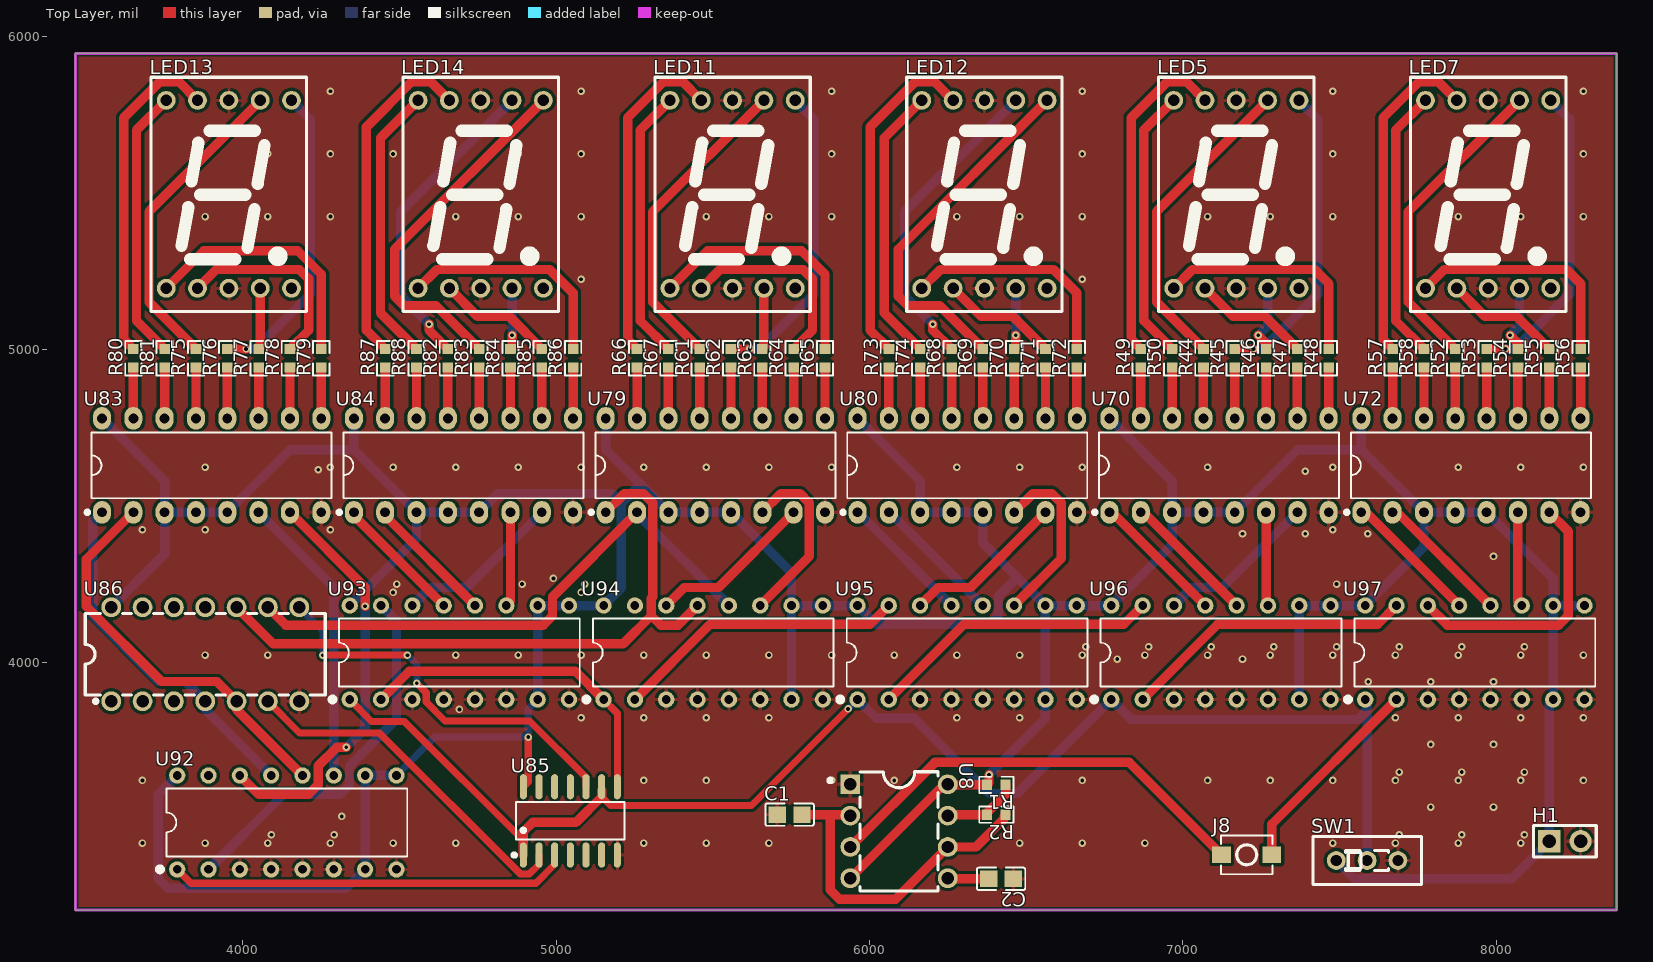
[diagram p0: Top Layer view]
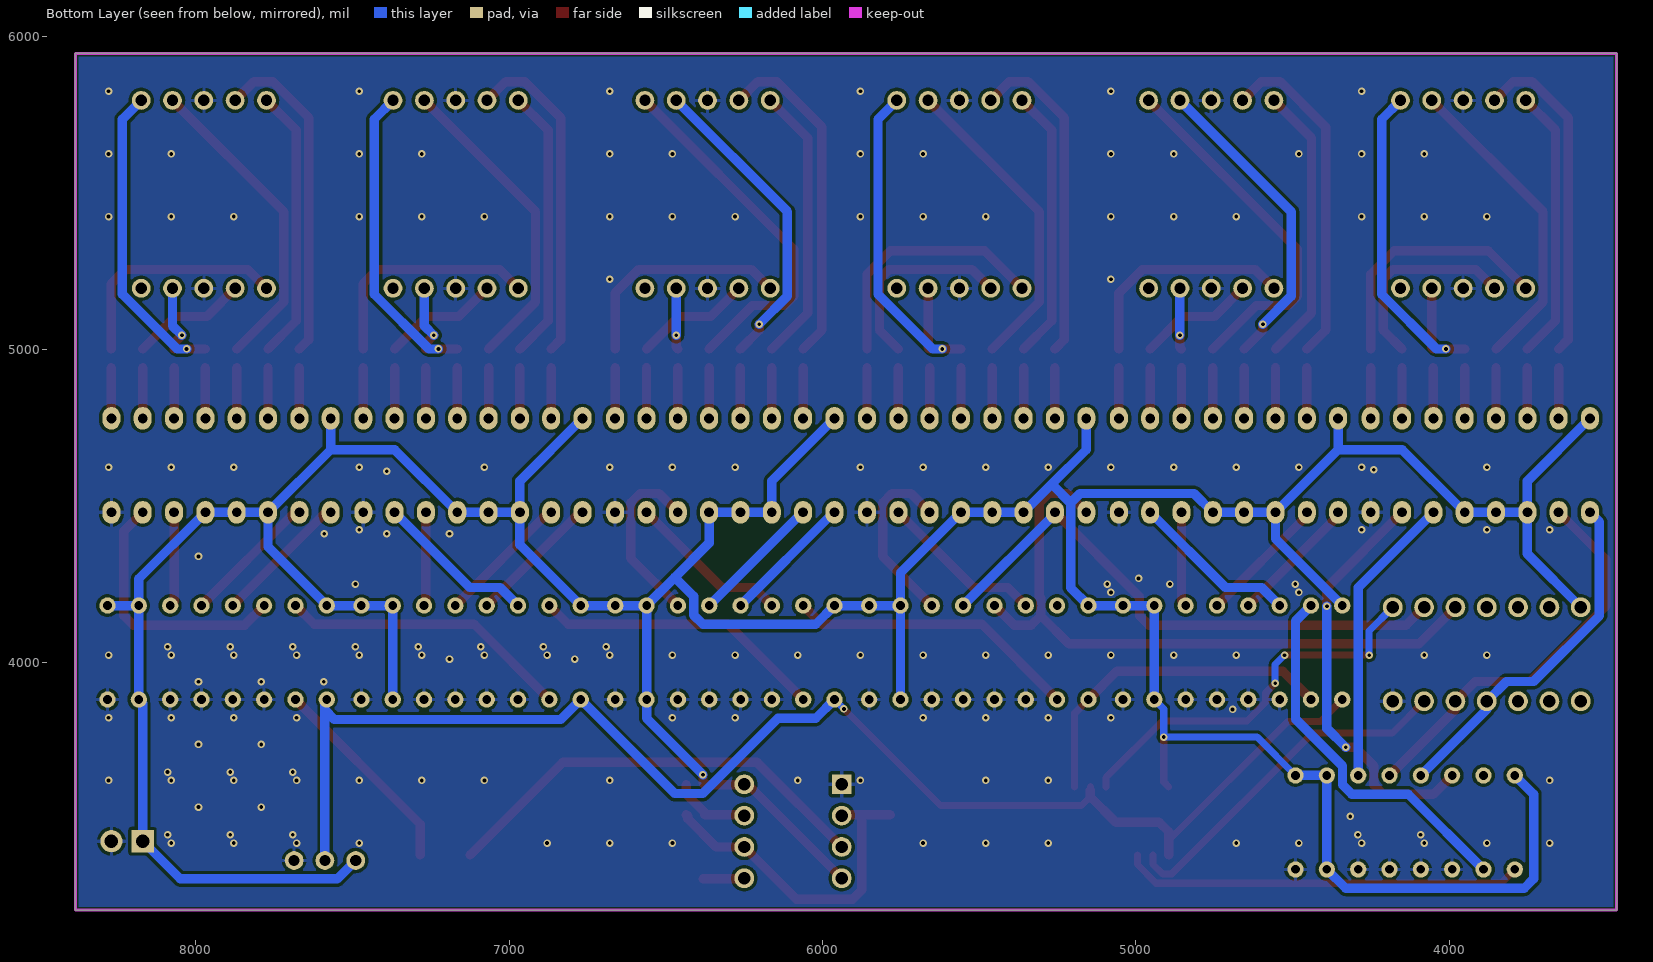
[diagram p1: Bottom Layer view, seen from below]
# Altium PCB MISC52151.pcbdoc
Units mil, origin at the board's own origin, x right, y up, seen from the top; angles counter-clockwise.
Board outline 4920 x 2735 mil, 2 copper layers (Top Layer, Bottom Layer), stack 62.206 mil thick; 70 components, 124 nets, 387 pads, 179 vias.

## Layer stack, top to bottom
Top Solder Mask Layer: solder mask 0.394, Dk 3.3
Top Layer: signal copper 1.379
Dielectric1: surface 59.449, FR4, Dk 4.5
Bottom Layer: signal copper 1.378
Bottom Solder Mask Layer: solder mask 0.394, Dk 3.3

## Board outline
3465,5945 3465,3210 8385,3210 8385,5945

## Design rules (kind name [scope] priority, off if disabled: settings)
BoardOutlineClearance copperThickness2oz_1 [All] p2 off: genericclearance=7.99 ignorepadtopadclearanceinfootprint=FALSE except(0: Arc-SplitContinuation Track-SplitContinuation SMDPad-SplitContinuation THPad-SplitContinuation Via-SplitContinuation Fill-SplitContinuation Region-SplitContinuation Poly-SplitContinuation Text-SplitContinuation Hole-SplitContinuation; 5.98: Arc-CutoutEdge Track-CutoutEdge SMDPad-CutoutEdge THPad-CutoutEdge Via-CutoutEdge Text-CutoutEdge; 6.89: Hole-OutlineEdge Hole-CutoutEdge; 10: Poly-OutlineEdge Poly-CutoutEdge; 11.81: Arc-OutlineEdge Track-OutlineEdge SMDPad-OutlineEdge THPad-OutlineEdge Via-OutlineEdge Fill-OutlineEdge Region-OutlineEdge Text-OutlineEdge Fill-CutoutEdge Region-CutoutEdge)
BoardOutlineClearance Plane_innerPlane_1 [All] p4 off: genericclearance=4.02 ignorepadtopadclearanceinfootprint=FALSE except(0: Arc-SplitContinuation Track-SplitContinuation SMDPad-SplitContinuation THPad-SplitContinuation Via-SplitContinuation Fill-SplitContinuation Region-SplitContinuation Poly-SplitContinuation Text-SplitContinuation Hole-SplitContinuation; 5.98: Arc-CutoutEdge Track-CutoutEdge SMDPad-CutoutEdge THPad-CutoutEdge Via-CutoutEdge Text-CutoutEdge; 6.89: Hole-OutlineEdge Hole-CutoutEdge; 10: Poly-OutlineEdge Poly-CutoutEdge; 11.81: Arc-OutlineEdge Track-OutlineEdge SMDPad-OutlineEdge THPad-OutlineEdge Via-OutlineEdge Fill-OutlineEdge Region-OutlineEdge Text-OutlineEdge Fill-CutoutEdge Region-CutoutEdge)
BoardOutlineClearance Copper_copperRegion_1 [All] p6 off: genericclearance=4.02 ignorepadtopadclearanceinfootprint=FALSE except(0: Arc-SplitContinuation Track-SplitContinuation SMDPad-SplitContinuation THPad-SplitContinuation Via-SplitContinuation Fill-SplitContinuation Region-SplitContinuation Poly-SplitContinuation Text-SplitContinuation Hole-SplitContinuation; 5.98: Arc-CutoutEdge Track-CutoutEdge SMDPad-CutoutEdge THPad-CutoutEdge Via-CutoutEdge Text-CutoutEdge; 6.89: Hole-OutlineEdge Hole-CutoutEdge; 10: Poly-OutlineEdge Poly-CutoutEdge; 11.81: Arc-OutlineEdge Track-OutlineEdge SMDPad-OutlineEdge THPad-OutlineEdge Via-OutlineEdge Fill-OutlineEdge Region-OutlineEdge Text-OutlineEdge Fill-CutoutEdge Region-CutoutEdge)
BoardOutlineClearance copperThickness1oz_1 [All] p8: genericclearance=4.02 ignorepadtopadclearanceinfootprint=FALSE except(0: Arc-SplitContinuation Track-SplitContinuation SMDPad-SplitContinuation THPad-SplitContinuation Via-SplitContinuation Fill-SplitContinuation Region-SplitContinuation Poly-SplitContinuation Text-SplitContinuation Hole-SplitContinuation; 5.98: Arc-CutoutEdge Track-CutoutEdge SMDPad-CutoutEdge THPad-CutoutEdge Via-CutoutEdge Text-CutoutEdge; 6.89: Hole-OutlineEdge Hole-CutoutEdge; 10: Poly-OutlineEdge Poly-CutoutEdge; 11.81: Arc-OutlineEdge Track-OutlineEdge SMDPad-OutlineEdge THPad-OutlineEdge Via-OutlineEdge Fill-OutlineEdge Region-OutlineEdge Text-OutlineEdge Fill-CutoutEdge Region-CutoutEdge)
Clearance copperThickness2oz [All] p1 off: gap=7.99 ignorepadtopadclearanceinfootprint=FALSE except(5.98: SMDPad-Track SMDPad-SMDPad THPad-Track SMDPad-THPad THPad-THPad Track-Via SMDPad-Via THPad-Via Via-Via Fill-SMDPad Region-SMDPad Fill-THPad Region-THPad Fill-Via Region-Via Fill-Fill Fill-Region Region-Region Arc-Track Arc-SMDPad Arc-THPad Arc-Via Fill-Arc Region-Arc Arc-Arc Text-Track SMDPad-Text Text-THPad Text-Via Fill-Text Region-Text Arc-Text Text-Text; 6.89: Hole-Track Hole-SMDPad Hole-THPad Hole-Via Fill-Hole Region-Hole Hole-Arc Hole-Text; 10: Poly-Track Poly-SMDPad Poly-THPad Poly-Via Poly-Fill Poly-Region Poly-Poly Poly-Arc Poly-Text Poly-Hole; 11.81: Fill-Track Region-Track)
Clearance Plane_innerPlane [All] p3 off: gap=4.02 ignorepadtopadclearanceinfootprint=FALSE except(5.98: SMDPad-Track SMDPad-SMDPad THPad-Track SMDPad-THPad THPad-THPad Track-Via SMDPad-Via THPad-Via Via-Via Fill-SMDPad Region-SMDPad Fill-THPad Region-THPad Fill-Via Region-Via Fill-Fill Fill-Region Region-Region Arc-Track Arc-SMDPad Arc-THPad Arc-Via Fill-Arc Region-Arc Arc-Arc Text-Track SMDPad-Text Text-THPad Text-Via Fill-Text Region-Text Arc-Text Text-Text; 6.89: Hole-Track Hole-SMDPad Hole-THPad Hole-Via Fill-Hole Region-Hole Hole-Arc Hole-Text; 10: Poly-Track Poly-SMDPad Poly-THPad Poly-Via Poly-Fill Poly-Region Poly-Poly Poly-Arc Poly-Text Poly-Hole; 11.81: Fill-Track Region-Track)
Clearance Copper_copperRegion [All] p5 off: gap=4.02 ignorepadtopadclearanceinfootprint=FALSE except(5.98: SMDPad-Track SMDPad-SMDPad THPad-Track SMDPad-THPad THPad-THPad Track-Via SMDPad-Via THPad-Via Via-Via Fill-SMDPad Region-SMDPad Fill-THPad Region-THPad Fill-Via Region-Via Fill-Fill Fill-Region Region-Region Arc-Track Arc-SMDPad Arc-THPad Arc-Via Fill-Arc Region-Arc Arc-Arc Text-Track SMDPad-Text Text-THPad Text-Via Fill-Text Region-Text Arc-Text Text-Text; 6.89: Hole-Track Hole-SMDPad Hole-THPad Hole-Via Fill-Hole Region-Hole Hole-Arc Hole-Text; 10: Poly-Track Poly-SMDPad Poly-THPad Poly-Via Poly-Fill Poly-Region Poly-Poly Poly-Arc Poly-Text Poly-Hole; 11.81: Fill-Track Region-Track)
Clearance copperThickness1oz [All] p7: gap=4.02 ignorepadtopadclearanceinfootprint=FALSE except(5.98: SMDPad-Track SMDPad-SMDPad THPad-Track SMDPad-THPad THPad-THPad Track-Via SMDPad-Via THPad-Via Via-Via Fill-SMDPad Region-SMDPad Fill-THPad Region-THPad Fill-Via Region-Via Fill-Fill Fill-Region Region-Region Arc-Track Arc-SMDPad Arc-THPad Arc-Via Fill-Arc Region-Arc Arc-Arc Text-Track SMDPad-Text Text-THPad Text-Via Fill-Text Region-Text Arc-Text Text-Text; 6.89: Hole-Track Hole-SMDPad Hole-THPad Hole-Via Fill-Hole Region-Hole Hole-Arc Hole-Text; 10: Poly-Track Poly-SMDPad Poly-THPad Poly-Via Poly-Fill Poly-Region Poly-Poly Poly-Arc Poly-Text Poly-Hole; 11.81: Fill-Track Region-Track)
DiffPairsRouting differentialPair [All] p1: maxlimit=6 minlimit=6 mostfreqgap=6 toplayer_minwidth=5 toplayer_prefwidth=10 toplayer_maxwidth=100 toplayer_mingap=6 toplayer_prefgap=6 toplayer_maxgap=6 bottomlayer_minwidth=5 bottomlayer_prefwidth=10 bottomlayer_maxwidth=100 bottomlayer_mingap=6 bottomlayer_prefgap=6 bottomlayer_maxgap=6 maxuncoupledlength=10
HoleToHoleClearance otherClearance [All] p1: gap=11.81 allowstackedmicrovias=TRUE
Length netLength [All] p1: minlimit=0 maxlimit=0
PasteMaskExpansion pasteMaskExpansion [All] p1: expansion=0
PlaneConnect innerPlane [All] p1: planeconnectstyle=Relief reliefexpansion=20 reliefentries=4 reliefconductorwidth=10 reliefairgap=10
PolygonConnect copperRegion [All] p1: connectstyle=Relief reliefconductorwidth=10 reliefentries=4 polygonreliefangle="90 Angle" airgapwidth=10 via.connectstyle=Relief via.reliefconductorwidth=10 via.reliefentries=4 via.polygonreliefangle="90 Angle" via.airgapwidth=10
RoutingVias viaSize [All] p1: holewidth=12.01 width=24.02 viastyle="Through Hole" minholewidth=11.81 minwidth=19.68 maxholewidth=248.03 maxwidth=393.7
SolderMaskExpansion solderMaskExpansion [IsVia] p1: expansion=-1000 istentingtop=TRUE
SolderMaskExpansion solderMaskExpansion [All] p2: expansion=2.01 istentingtop=FALSE
Width copperThickness2oz_2 [All] p1 off: maxlimit=100 minlimit=8 preferedwidth=10
Width copperThickness1oz_2 [All] p2: maxlimit=100 minlimit=5 preferedwidth=30

## Components (designator, comment, footprint, x,y, rotation, side; value= is the part's Value field where it differs from the comment)
C1 "1uF" C0805 5745,3515 r0 top
C2 "10nF" C0805 6420,3310 r180 top
H1 "" HDR-TH_2P-P2.54-V-M-1 8220,3430 r0 top
J8 "轻触按键3*4*H" SW-SMD_L4.0-W2.9-LS5.0 7204.15,3386.7 r0 top
LED5 "" LED-SEG-TH_10P-L12.6-W19.0-P2.54-S15.24-BL 7170.99,5495 r0 top
LED7 "" LED-SEG-TH_10P-L12.6-W19.0-P2.54-S15.24-BL 7975,5495 r0 top
LED11 "" LED-SEG-TH_10P-L12.6-W19.0-P2.54-S15.24-BL 5562.96,5495 r0 top
LED12 "" LED-SEG-TH_10P-L12.6-W19.0-P2.54-S15.24-BL 6366.98,5495 r0 top
LED13 "" LED-SEG-TH_10P-L12.6-W19.0-P2.54-S15.24-BL 3954.94,5495 r0 top
LED14 "" LED-SEG-TH_10P-L12.6-W19.0-P2.54-S15.24-BL 4758.95,5495 r0 top
R1 "10k" R0603 6405,3610 r180 top
R2 "2.2k" R0603 6405,3515 r180 top
R44 "250" R0603 7066.04,4971.74 r90 top
R45 "250" R0603 7166.03,4971.74 r90 top
R46 "250" R0603 7266.02,4971.74 r90 top
R47 "250" R0603 7366,4971.74 r90 top
R48 "250" R0603 7465.99,4971.74 r90 top
R49 "250" R0603 6866.07,4971.74 r90 top
R50 "250" R0603 6966.06,4971.74 r90 top
R52 "250" R0603 7870.06,4971.74 r90 top
R53 "250" R0603 7970.04,4971.74 r90 top
R54 "250" R0603 8070.03,4971.74 r90 top
R55 "250" R0603 8170.01,4971.74 r90 top
R56 "250" R0603 8270,4971.74 r90 top
R57 "250" R0603 7670.09,4971.74 r90 top
R58 "250" R0603 7770.07,4971.74 r90 top
R61 "250" R0603 5458.02,4971.74 r90 top
R62 "250" R0603 5558.01,4971.74 r90 top
R63 "250" R0603 5657.99,4971.74 r90 top
R64 "250" R0603 5757.98,4971.74 r90 top
R65 "250" R0603 5857.96,4971.74 r90 top
R66 "250" R0603 5258.05,4971.74 r90 top
R67 "250" R0603 5358.04,4971.74 r90 top
R68 "250" R0603 6262.03,4971.74 r90 top
R69 "250" R0603 6362.02,4971.74 r90 top
R70 "250" R0603 6462,4971.74 r90 top
R71 "250" R0603 6561.99,4971.74 r90 top
R72 "250" R0603 6661.98,4971.74 r90 top
R73 "250" R0603 6062.06,4971.74 r90 top
R74 "250" R0603 6162.05,4971.74 r90 top
R75 "250" R0603 3850,4971.74 r90 top
R76 "250" R0603 3949.98,4971.74 r90 top
R77 "250" R0603 4049.97,4971.74 r90 top
R78 "250" R0603 4149.95,4971.74 r90 top
R79 "250" R0603 4249.94,4971.74 r90 top
R80 "250" R0603 3650.03,4971.74 r90 top
R81 "250" R0603 3750.01,4971.74 r90 top
R82 "250" R0603 4654.01,4971.74 r90 top
R83 "250" R0603 4753.99,4971.74 r90 top
R84 "250" R0603 4853.98,4971.74 r90 top
R85 "250" R0603 4953.97,4971.74 r90 top
R86 "250" R0603 5053.95,4971.74 r90 top
R87 "250" R0603 4454.04,4971.74 r90 top
R88 "250" R0603 4554.02,4971.74 r90 top
SW1 "开关" SW-TH_SS-12D01-GX 7588.45,3368.51 r0 top
U8 "NE555PE4" PDIP-8_L9.6-W6.4-P2.54-LS7.9-BL-1 6094.24,3461.7 r270 top
U70 "SN74LS48N" DIP-16_L19.3-W6.4-P2.54-LS7.6-BL 7115.99,4630 r0 top
U72 "SN74LS48N" DIP-16_L19.3-W6.4-P2.54-LS7.6-BL 7920,4630 r0 top
U79 "SN74LS48N" DIP-16_L19.3-W6.4-P2.54-LS7.6-BL 5507.96,4630 r0 top
U80 "SN74LS48N" DIP-16_L19.3-W6.4-P2.54-LS7.6-BL 6311.98,4630 r0 top
U83 "SN74LS48N" DIP-16_L19.3-W6.4-P2.54-LS7.6-BL 3899.94,4630 r0 top
U84 "SN74LS48N" DIP-16_L19.3-W6.4-P2.54-LS7.6-BL 4703.95,4630 r0 top
U85 "SN74LS08DR(LX)" SOIC-14_L8.7-W3.9-P1.27-LS6.0-BL 5045,3495 r0 top
U86 "SN74LS00N(LX)" PDIP-14_L19.3-W6.4-P2.54-LS7.9-BL 3879.59,4026.83 r0 top
U92 "SN74LS160N(LX)" DIP-16_L19.4-W6.4-P2.54-S7.6-BL 4140,3490 r0 top
U93 "SN74LS160N(LX)" DIP-16_L19.4-W6.4-P2.54-S7.6-BL 4690.73,4032.34 r0 top
U94 "SN74LS160N(LX)" DIP-16_L19.4-W6.4-P2.54-S7.6-BL 5501.15,4032.34 r0 top
U95 "SN74LS160N(LX)" DIP-16_L19.4-W6.4-P2.54-S7.6-BL 6311.56,4032.34 r0 top
U96 "SN74LS160N(LX)" DIP-16_L19.4-W6.4-P2.54-S7.6-BL 7121.97,4032.34 r0 top
U97 "SN74LS160N(LX)" DIP-16_L19.4-W6.4-P2.54-S7.6-BL 7932.39,4032.34 r0 top

## Footprints (in the part's own frame and the unit in brackets; to place one, negate y for a bottom-side part, rotate by r counter-clockwise, add the part's x,y. Pads: shape width x height; smd on the part's side, far side on the other; paste and mask are expansions set on the pad)
C0805 [mm]
  rect 1.41x1.35 smd paste-100 mask+0.051: 1(-1,0) 2(1,0)
  silkscreen extent -1.96,-0.9 1.96,0.9
DIP-16_L19.3-W6.4-P2.54-LS7.6-BL [mm]
  oval 1.46x1.825 hole 0.8: 1(-8.89,-3.81) 2(-6.35,-3.81) 3(-3.81,-3.81) 4(-1.27,-3.81) 5(1.27,-3.81) 6(3.81,-3.81) 7(6.35,-3.81) 8(8.89,-3.81) 9(8.89,3.81) 10(6.35,3.81) 11(3.81,3.81) 12(1.27,3.81) 13(-1.27,3.81) 14(-3.81,3.81) 15(-6.35,3.81) 16(-8.89,3.81)
  silkscreen extent -10.22,-3.96 9.73,2.67
DIP-16_L19.4-W6.4-P2.54-S7.6-BL [mm]
  round 1.32 hole 0.7: 1(-8.89,-3.81) 2(-6.35,-3.81) 3(-3.81,-3.81) 4(-1.27,-3.81) 5(1.27,-3.81) 6(3.81,-3.81) 7(6.35,-3.81) 8(8.89,-3.81) 9(8.89,3.81) 10(6.35,3.81) 11(3.81,3.81) 12(1.27,3.81) 13(-1.27,3.81) 14(-3.81,3.81) 15(-6.35,3.81) 16(-8.89,3.81)
  silkscreen extent -10.49,-4 9.76,2.76
HDR-TH_2P-P2.54-V-M-1 [mm]
  rect 1.8x1.8 hole 1.1: 1(-1.27,0)
  round 1.8 hole 1.1: 2(1.27,0)
  silkscreen extent -2.54,-1.27 2.54,1.27
LED-SEG-TH_10P-L12.6-W19.0-P2.54-S15.24-BL [mil]
  round 60 hole 36: 1(-200,-300) 2(-100,-300) 3(0,-300) 4(100,-300) 5(200,-300) 6(200,300) 7(100,300) 8(0,300) 9(-100,300) 10(-200,300)
  silkscreen extent -248,-374 248,374
PDIP-8_L9.6-W6.4-P2.54-LS7.9-BL-1 [mil]
  rect 63x63 hole 39.37: 1(-150,-155.51)
  round 63 hole 39.37: 2(-50,-155.51) 3(50,-155.51) 4(150,-155.51) 5(150,155.52) 6(50,155.52) 7(-50,155.52) 8(-150,155.52)
  silkscreen extent -190,-226 190,125
PDIP-14_L19.3-W6.4-P2.54-LS7.9-BL [mm]
  round 1.6 hole 1: 1(-7.62,-3.81) 2(-5.08,-3.81) 3(-2.54,-3.81) 4(0,-3.81) 5(2.54,-3.81) 6(5.08,-3.81) 7(7.62,-3.81) 8(7.62,3.81) 9(5.08,3.81) 10(2.54,3.81) 11(0,3.81) 12(-2.54,3.81) 13(-5.08,3.81) 14(-7.62,3.81)
  silkscreen extent -9.73,-3.96 9.73,3.3
R0603 [mil]
  rect 31.75x34.02 smd paste-3937.01 mask+2: 1(-29.66,0) 2(29.66,0)
  silkscreen extent -55,-26 55,26
SOIC-14_L8.7-W3.9-P1.27-LS6.0-BL [mil]
  oval 22.6x80.24 smd: 1(-150,-109.02) 2(-100,-109.02) 3(-50,-109.02) 4(0,-109.02) 5(50,-109.02) 6(100,-109.02) 7(150,-109.02) 8(150,109.02) 9(100,109.02) 10(50,109.02) 11(0,109.02) 12(-50,109.02) 13(-100,109.02) 14(-150,109.02)
  silkscreen extent -185,-115 173,60
SW-SMD_L4.0-W2.9-LS5.0 [mm]
  rect 1.53x1.36 smd: 1(-2.035,0) 2(2.035,0)
  silkscreen extent -2.08,-1.58 2.08,1.58
SW-TH_SS-12D01-GX [mil]
  round 60 hole 36: 1(-98.43,0) 2(-0.01,0) 3(98.42,0)
  silkscreen extent -173,-77 173,77

## Via types
v1: diameter 24.02, hole 12, Top Layer to Bottom Layer, 179 vias

## Nets (pads, with @x,y where several pads share a name; then routed paths per layer and width w, separated by ;. In a path a pad name is that pad's centre, name@x,y a point inside that pad or via, vN(x,y) a via of type N, cw(c..) or ccw(c..) an arc to the next point about the centre after c; other vN are vias at no path point)
$1N38628: U70.7 U96.14 | length 517.3
  Bottom Layer w30: U96.14 7029.63,4240 7125.99,4240 U70.7
$1N38636: U70.1 U96.13 | length 429.3
  Top Layer w30: U70.1 6774.32,4480 U96.13
$1N38644: U70.2 U96.12 | length 429.3
  Top Layer w30: U70.2 6874.32,4480 U96.12
$1N38648: U70.6 U96.11 | length 300.1
  Top Layer w30: U70.6 7265.99,4188.33 U96.11
$1N39456: U72.7 U97.14 | length 840.7
  Top Layer w30: U97.14 7844.73,4120 8200,4120 8230,4150 8230,4420 U72.7
$1N39468: U72.6 U97.11 | length 302.8
  Top Layer w30: U72.6 8070,4194.73 U97.11
$1N58076: R1.1 R2.2 U8.7 | length 246.5
  Top Layer w30: U8.7@6249.75,3511.7 6253.04,3515 R2.2 6375.34,3520.68 6434.66,3580 R1.1
$1N58077: C1.2 R2.1 U8.2 U8.6 | length 1085.2
  Top Layer w30: C1.2 5874.37,3515 ; U8.2 5935.43,3515 5874.37,3515 ; R2.1 6429.75,3510.09 6429.75,3501.7 6339.75,3411.7 6249.75,3411.7 6083.04,3245 5904.37,3245 5874.37,3275 5874.37,3515
$1N58078: C2.2 U8.5 | length 131.6
  Top Layer w30: U8.5@6249.75,3311.7 6251.45,3310 C2.2
$1N58085: J8.1 U8.3 | length 1419.3
  Top Layer w30: U8.3 6208.73,3681.7 6829.03,3681.7 J8.1
$1N58825: LED5.7 R44.2 | length 1002.8
  Top Layer w30: R44.2 6916.04,5151.4 6916.04,5440.06 LED5.7
$1N58826: LED5.6 R45.2 | length 980.9
  Top Layer w30: R45.2 v1(7226.03,5001.4)
  Bottom Layer w30: v1(7226.03,5001.4) 7256.03,5001.4 7430.99,5176.36 7430.99,5735 LED5.6
$1N58827: LED5.4 R46.2 | length 216.4
  Top Layer w30: v1(7240.99,5045) 7266.02,5019.97 R46.2
  Bottom Layer w30: v1(7240.99,5045) 7270.99,5075 LED5.4
$1N58828: LED5.2 R47.2 | length 375.2
  Top Layer w30: LED5.2 7160.99,5105 7262.4,5105 R47.2
$1N58829: LED5.1 R48.2 | length 747.1
  Top Layer w30: LED5.1 7030.99,5255 7420.99,5255 7465.99,5210 R48.2
$1N58830: LED5.9 R49.2 | length 1058.5
  Top Layer w30: R49.2 6836.07,5031.4 6836.07,5740.09 6950.99,5855 7010.99,5855 LED5.9
$1N58831: LED5.10 R50.2 | length 870.2
  Top Layer w30: R50.2 6876.06,5091.4 6876.06,5700.07 LED5.10
$1N58832: R44.1 U70.13 | length 162
  Top Layer w30: U70.13@7066.04,4780.06 R44.1
$1N58833: R45.1 U70.12 | length 162
  Top Layer w30: U70.12 R45.1
$1N58834: R46.1 U70.11 | length 162.1
  Top Layer w30: U70.11 R46.1
$1N58835: R47.1 U70.10 | length 162.1
  Top Layer w30: U70.10 R47.1
$1N58836: R48.1 U70.9 | length 162.1
  Top Layer w30: U70.9 R48.1
$1N58837: R49.1 U70.15 | length 162
  Top Layer w30: U70.15@6866.07,4780.09 R49.1
$1N58838: R50.1 U70.14 | length 162
  Top Layer w30: U70.14@6966.06,4780.07 R50.1
$1N58846: LED7.7 R52.2 | length 1002.8
  Top Layer w30: R52.2 7720.06,5151.4 7720.06,5440.06 LED7.7
$1N58847: LED7.6 R53.2 | length 980.9
  Top Layer w30: R53.2 v1(8030.04,5001.4)
  Bottom Layer w30: v1(8030.04,5001.4) 8060.04,5001.4 8235,5176.36 8235,5735 LED7.6
$1N58848: LED7.4 R54.2 | length 216.4
  Top Layer w30: v1(8045,5045) 8070.03,5019.97 R54.2
  Bottom Layer w30: v1(8045,5045) 8075,5075 LED7.4
$1N58849: LED7.2 R55.2 | length 375.2
  Top Layer w30: LED7.2 7965,5105 8066.41,5105 R55.2
$1N58850: LED7.1 R56.2 | length 747.1
  Top Layer w30: LED7.1 7835,5255 8225,5255 8270,5210 R56.2
$1N58851: LED7.9 R57.2 | length 1058.5
  Top Layer w30: R57.2 7640.09,5031.4 7640.09,5740.09 7755,5855 7815,5855 LED7.9
$1N58852: LED7.10 R58.2 | length 870.2
  Top Layer w30: R58.2 7680.07,5091.4 7680.07,5700.07 LED7.10
$1N58853: R52.1 U72.13 | length 162
  Top Layer w30: U72.13@7870.06,4780.06 R52.1
$1N58854: R53.1 U72.12 | length 162
  Top Layer w30: U72.12 R53.1
$1N58855: R54.1 U72.11 | length 162.1
  Top Layer w30: U72.11 R54.1
$1N58856: R55.1 U72.10 | length 162.1
  Top Layer w30: U72.10 R55.1
$1N58857: R56.1 U72.9 | length 162.1
  Top Layer w30: U72.9 R56.1
$1N58858: R57.1 U72.15 | length 162
  Top Layer w30: U72.15@7670.09,4780.09 R57.1
$1N58859: R58.1 U72.14 | length 162
  Top Layer w30: U72.14@7770.07,4780.07 R58.1
$1N59894: R74.1 U80.14 | length 162
  Top Layer w30: U80.14@6162.05,4780.07 R74.1
$1N59895: R71.1 U80.10 | length 162.1
  Top Layer w30: U80.10 R71.1
$1N59896: R70.1 U80.11 | length 162.1
  Top Layer w30: U80.11 R70.1
$1N59897: R69.1 U80.12 | length 162
  Top Layer w30: U80.12 R69.1
$1N59898: R72.1 U80.9 | length 162.1
  Top Layer w30: U80.9 R72.1
$1N59899: R73.1 U80.15 | length 162
  Top Layer w30: U80.15@6062.06,4780.09 R73.1
$1N59900: R68.1 U80.13 | length 162
  Top Layer w30: U80.13@6262.03,4780.06 R68.1
$1N59901: LED12.4 R70.2 | length 195.7
  Top Layer w30: R70.2 6466.98,5006.37 v1(6466.98,5045)
  Bottom Layer w30: v1(6466.98,5045) LED12.4
$1N59902: LED12.2 R71.2 | length 375.2
  Top Layer w30: LED12.2 6356.98,5105 6458.39,5105 R71.2
$1N59903: LED12.10 R74.2 | length 891
  Top Layer w30: R74.2 6046.98,5116.47 6046.98,5675 LED12.10
$1N59904: LED12.1 R72.2 | length 729.5
  Top Layer w30: LED12.1 6226.98,5255 6586.98,5255 6661.98,5180 R72.2
$1N59905: LED12.9 R73.2 | length 1083.3
  Top Layer w30: R73.2 6002.06,5061.4 6002.06,5710.09 6146.98,5855 6206.98,5855 LED12.9
$1N59906: LED12.6 R69.2 | length 1161.5
  Top Layer w30: R69.2 6223.38,5140.04 6122.02,5140.04 6092.02,5170.04 6092.02,5320.04 LED12.6
$1N59907: LED12.7 R68.2 | length 1002.8
  Top Layer w30: v1(6202.03,5080.06) 6202.03,5061.4 R68.2
  Bottom Layer w30: v1(6202.03,5080.06) 6112.03,5170.06 6112.03,5440.06 LED12.7
$1N59910: R61.1 U79.13 | length 162
  Top Layer w30: U79.13@5458.02,4780.06 R61.1
$1N59911: R62.1 U79.12 | length 162
  Top Layer w30: U79.12 R62.1
$1N59912: R66.1 U79.15 | length 162
  Top Layer w30: U79.15@5258.05,4780.09 R66.1
$1N59913: R67.1 U79.14 | length 162
  Top Layer w30: U79.14@5358.04,4780.07 R67.1
$1N59914: R65.1 U79.9 | length 162.1
  Top Layer w30: U79.9 R65.1
$1N59915: R64.1 U79.10 | length 162.1
  Top Layer w30: U79.10 R64.1
$1N59916: R63.1 U79.11 | length 162.1
  Top Layer w30: U79.11 R63.1
$1N59917: LED11.7 R61.2 | length 1002.8
  Top Layer w30: R61.2 5308.02,5151.4 5308.02,5440.06 LED11.7
$1N59918: LED11.6 R62.2 | length 980.9
  Top Layer w30: R62.2 v1(5618.01,5001.4)
  Bottom Layer w30: v1(5618.01,5001.4) 5648.01,5001.4 5822.96,5176.36 5822.96,5735 LED11.6
$1N59919: LED11.10 R67.2 | length 870.2
  Top Layer w30: R67.2 5268.04,5091.4 5268.04,5700.07 LED11.10
$1N59920: LED11.4 R63.2 | length 195.7
  Top Layer w30: R63.2 5662.96,5006.37 LED11.4
$1N59921: LED11.2 R64.2 | length 640.7
  Top Layer w30: LED11.2 5522.96,5255 5787.98,5255 5817.98,5225 5817.98,5061.4 R64.2
$1N59922: LED11.1 R65.2 | length 814.4
  Top Layer w30: LED11.1 5482.96,5315 5782.96,5315 5857.96,5240 R65.2
$1N59923: LED11.9 R66.2 | length 1058.5
  Top Layer w30: R66.2 5228.05,5031.4 5228.05,5740.09 5342.96,5855 5402.96,5855 LED11.9
$1N59924: U80.6 U95.11 | length 577.2
  Top Layer w30: U95.11 6611.98,4332.76 6611.98,4510 6581.98,4540 6521.98,4540 U80.6
$1N59936: U80.1 U95.13 | length 422.9
  Bottom Layer w30: U80.1 5963.9,4480 U95.13
$1N60930: R88.1 U84.14 | length 162
  Top Layer w30: U84.14@4554.02,4780.07 R88.1
$1N60931: R85.1 U84.10 | length 162.1
  Top Layer w30: U84.10 R85.1
$1N60932: R84.1 U84.11 | length 162.1
  Top Layer w30: U84.11 R84.1
$1N60933: R83.1 U84.12 | length 162
  Top Layer w30: U84.12 R83.1
$1N60934: R86.1 U84.9 | length 162.1
  Top Layer w30: U84.9 R86.1
$1N60935: R87.1 U84.15 | length 162
  Top Layer w30: U84.15@4454.04,4780.09 R87.1
$1N60936: R82.1 U84.13 | length 162
  Top Layer w30: U84.13@4654.01,4780.06 R82.1
$1N60937: LED14.4 R84.2 | length 195.7
  Top Layer w30: R84.2 4858.95,5006.37 v1(4858.95,5045)
  Bottom Layer w30: v1(4858.95,5045) LED14.4
$1N60938: LED14.2 R85.2 | length 375.2
  Top Layer w30: LED14.2 4748.95,5105 4850.37,5105 R85.2
$1N60939: LED14.10 R88.2 | length 891
  Top Layer w30: R88.2 4438.95,5116.47 4438.95,5675 LED14.10
$1N60940: LED14.1 R86.2 | length 729.5
  Top Layer w30: LED14.1 4618.95,5255 4978.95,5255 5053.95,5180 R86.2
$1N60941: LED14.9 R87.2 | length 1083.3
  Top Layer w30: R87.2 4394.04,5061.4 4394.04,5710.09 4538.95,5855 4598.95,5855 LED14.9
$1N60942: LED14.6 R83.2 | length 1161.5
  Top Layer w30: R83.2 4615.35,5140.04 4513.99,5140.04 4483.99,5170.04 4483.99,5320.04 LED14.6
$1N60943: LED14.7 R82.2 | length 1002.8
  Top Layer w30: v1(4594.01,5080.06) 4594.01,5061.4 R82.2
  Bottom Layer w30: v1(4594.01,5080.06) 4504.01,5170.06 4504.01,5440.06 LED14.7
$1N60946: R75.1 U83.13 | length 162
  Top Layer w30: U83.13@3850,4780.06 R75.1
$1N60947: R76.1 U83.12 | length 162
  Top Layer w30: U83.12@3949.98,4780.04 R76.1
$1N60948: R80.1 U83.15 | length 162
  Top Layer w30: U83.15@3650.03,4780.09 R80.1
$1N60949: R81.1 U83.14 | length 162
  Top Layer w30: U83.14@3750.01,4780.07 R81.1
$1N60950: R79.1 U83.9 | length 162.1
  Top Layer w30: U83.9 R79.1
$1N60951: R78.1 U83.10 | length 162.1
  Top Layer w30: U83.10@4149.95,4780.01 R78.1
$1N60952: R77.1 U83.11 | length 162.1
  Top Layer w30: U83.11@4049.97,4780.03 R77.1
$1N60953: LED13.7 R75.2 | length 1002.8
  Top Layer w30: R75.2 3700,5151.4 3700,5440.06 LED13.7
$1N60954: LED13.6 R76.2 | length 980.9
  Top Layer w30: R76.2 v1(4009.98,5001.4)
  Bottom Layer w30: v1(4009.98,5001.4) 4039.98,5001.4 4214.94,5176.36 4214.94,5735 LED13.6
$1N60955: LED13.10 R81.2 | length 870.2
  Top Layer w30: R81.2 3660.01,5091.4 3660.01,5700.07 LED13.10
$1N60956: LED13.4 R77.2 | length 195.7
  Top Layer w30: R77.2 4054.94,5006.37 LED13.4
$1N60957: LED13.2 R78.2 | length 640.7
  Top Layer w30: LED13.2 3914.94,5255 4179.95,5255 4209.95,5225 4209.95,5061.4 R78.2
$1N60958: LED13.1 R79.2 | length 814.4
  Top Layer w30: LED13.1 3874.94,5315 4174.94,5315 4249.94,5240 R79.2
$1N60959: LED13.9 R80.2 | length 1058.5
  Top Layer w30: R80.2 3620.03,5031.4 3620.03,5740.09 3734.94,5855 3794.94,5855 LED13.9
$1N60968: U84.7 U93.14 | length 536.5
  Bottom Layer w30: U93.14 4598.39,4240 4713.95,4240 U84.7
$1N60972: U84.1 U93.13 | length 416.4
  Top Layer w30: U84.1 4353.95,4469.12 U93.13
$1N60991: U83.7 U92.14 | length 1336.3
  Top Layer w30: U92.14 4050,3580 4209.94,3580 4239.94,3610 4239.94,3670 4299.94,3730 v1(4329.94,3730) ; U83.7 4389.94,4240 v1(4389.94,4180)
  Bottom Layer w30: v1(4329.94,3730) 4389.94,3790 v1(4389.94,4180)
$1N60995: U83.6 U92.11 | length 939.4
  Bottom Layer w30: U83.6 4290,4239.94 U92.11
$1N65984: J8.2 U97.2 | length 660.5
  Top Layer w30: J8.2 7284.27,3484.23 U97.2
$1N66441: U85.2 U86.6 | length 1136
  Top Layer w22.6: U86.6 4180.45,3775.98 4435,3775.98 4885,3325.98 4915,3325.98 4945,3355.98 U85.2
$1N66593: U85.10 U86.8 | length 1268.3
  Top Layer w22.6: v1(4255,4024.02) v1(4525,4024.02) ; v1(4555,3934.02) 4585,3904.02 4585,3874.02 4645,3814.02 4915,3814.02 5095,3634.02 U85.10
  Bottom Layer w22.6: U86.8 4255,4101.43 v1(4255,4024.02) ; v1(4525,4024.02) 4555,3994.02 v1(4555,3934.02)
$1N66598: U85.8 U93.2 U94.1 | length 1081.5
  Top Layer w22.6: U94.1 5195,3838.49 U85.8
  Top Layer w30: U93.2 4530.73,3972.34 5061.15,3972.34 U94.1
$1N66613: SW1.2 U85.1 U85.9 U93.1 U95.1 U96.1 U97.1 | length 4542
  Top Layer w22.6: U93.1 4410.82,3812.25 4515,3812.25 4895,3432.25 ; U85.9@5145,3572.25 5173.23,3544.02 5623.23,3544.02 v1(5931.56,3852.34) ; U85.9@5145,3591.99 U85.9
  Top Layer w30: U85.1 4895,3432.25 4895,3460 4925,3490 5062.75,3490 5145,3572.25 U85.9@5145,3591.99
  Bottom Layer w22.6: v1(5931.56,3852.34) U95.1
  Bottom Layer w30: U95.1 6021.56,3822.34 6141.97,3822.34 6381.97,3582.34 6471.97,3582.34 U96.1 6835.81,3818.51 7558.44,3818.51 7588.44,3848.51 ; U97.1 7588.44,3876.29 7588.44,3848.51 ; SW1.2 7588.44,3848.51
$1N70339: U85.3 U92.1 | length 1278.1
  Top Layer w22.6: U92.1 3834.02,3295.98 4935,3295.98 4995,3355.98 U85.3
$1N76513: U83.1 U86.4 U92.13 | length 1139.2
  Bottom Layer w30: U83.1 3519.94,4450 3519.94,4150 3729.94,3940 3816.43,3940 U86.4 3879.59,3850.41 U92.13
$1N76520: U83.2 U86.5 U92.12 | length 1291.3
  Top Layer w30: U83.2 3499.94,4330 3499.94,4180 3739.94,3940 3916.43,3940 U86.5 3979.59,3850.41 U92.12
$1N77124: U84.2 U93.12 | length 416.4
  Top Layer w30: U84.2 4453.95,4469.12 U93.12
$1N77129: U84.6 U93.11 | length 303.1
  Top Layer w30: U93.11 4853.95,4195.56 U84.6
$1N77482: U92.2 U93.15 | length 1216.7
  Bottom Layer w30: U92.2 4130,3580 4310,3580 4340,3610 4340,3670 4490,3820 4490,4133.07 U93.15
$1N77894: U79.1 U86.10 U94.13 | length 2144.6
  Top Layer w30: U86.10 4096.43,4060 5213.49,4060 5303.49,4150 ; U79.1 5217.96,4540 5277.96,4540 5307.96,4510 5307.96,4210 5303.49,4205.52 5303.49,4150 ; U94.13 5388.8,4120 5333.49,4120 5303.49,4150
$1N77913: U79.7 U94.14 | length 530.1
  Top Layer w30: U94.14 5408.8,4240 5517.96,4240 U79.7
$1N77936: U79.2 U86.9 U94.12 | length 1805.3
  Top Layer w30: U86.9 4136.43,4120 4957.96,4120 4987.96,4150 4987.96,4210 U79.2
  Bottom Layer w30: U79.2 5257.96,4475.52 U94.12
$1N77940: U79.6 U94.11 | length 579.9
  Top Layer w30: U94.11 5807.96,4339.16 5807.96,4510 5777.96,4540 5717.96,4540 U79.6
$1N78335: U80.7 U95.14 | length 523.7
  Top Layer w30: U95.14 6219.22,4240 6321.98,4240 U80.7
$1N78347: U80.2 U95.12 | length 422.9
  Bottom Layer w30: U80.2 6063.9,4480 U95.12
$1N78544: U94.2 U95.15 | length 934.7
  Top Layer w30: U94.2 5491.15,4122.34 6001.56,4122.34 U95.15
$1N78919: U72.1 U97.13 | length 435.7
  Top Layer w30: U72.1 7584.73,4480 U97.13
$1N78927: U72.2 U97.12 | length 435.7
  Top Layer w30: U72.2 7684.73,4480 U97.12
$1N79073: U96.2 U97.15 | length 934.7
  Top Layer w30: U96.2 7111.97,4122.34 7622.39,4122.34 U97.15
$1N81903: U95.2 U96.15 | length 934.7
  Top Layer w30: U95.2 6301.56,4122.34 6811.97,4122.34 U96.15
GND: C1.1 C2.1 H1.2 LED5.3 LED5.8 LED7.3 LED7.8 LED11.3 LED11.8 LED12.3 LED12.8 LED13.3 LED13.8 LED14.3 LED14.8 SW1.3 U8.1 U70.8 U72.8 U79.8 U80.8 U83.8 U84.8 U85.7 U86.7 U92.3 U92.4 U92.5 U92.6 U92.8 U93.3 U93.4 U93.5 U93.6 U93.8 U94.3 U94.4 U94.5 U94.6 U94.8 U95.3 U95.4 U95.5 U95.6 U95.8 U96.3 U96.4 U96.5 U96.6 U96.8 U97.3 U97.4 U97.5 U97.6 U97.8
  other v1: 3679.1,3424.1 3879.1,3424.1 4079.1,3424.1 4279.1,3424.1 4479.1,3424.1 4679.1,3424.1 5279.1,3424.1 5479.1,3424.1 5679.1,3424.1 6479.1,3424.1 6679.1,3424.1 6879.1,3424.1 7479.1,3424.1 7679.1,3424.1 7879.1,3424.1 8079.1,3424.1 4090.84,3450.9 4290.84,3450.9 7690.84,3450.9 7890.84,3450.9 8090.84,3450.9 4315.53,3509.1 7791.98,3539.1 7991.98,3539.1 3679.1,3624.1 5279.1,3624.1 5479.1,3624.1 5879.1,3624.1 6079.1,3624.1 6679.1,3624.1 7079.1,3624.1 7279.1,3624.1 7479.1,3624.1 7679.1,3624.1 7879.1,3624.1 8079.1,3624.1 8279.1,3624.1 7690.84,3650.9 7890.84,3650.9 8090.84,3650.9 7791.98,3739.1 7991.98,3739.1 5079.1,3824.1 5279.1,3824.1 5479.1,3824.1 5679.1,3824.1 6279.1,3824.1 6479.1,3824.1 7679.1,3824.1 7879.1,3824.1 8079.1,3824.1 8279.1,3824.1 4690.84,3850.9 7591.98,3939.1 7791.98,3939.1 7991.98,3939.1 6790.74,4011.44 7190.74,4011.44 3879.1,4024.1 4079.1,4024.1 4679.1,4024.1 4879.1,4024.1 5079.1,4024.1 5279.1,4024.1 5479.1,4024.1 5679.1,4024.1 5879.1,4024.1 6079.1,4024.1 6279.1,4024.1 6479.1,4024.1 6679.1,4024.1 6879.1,4024.1 7079.1,4024.1 7279.1,4024.1 7479.1,4024.1 7679.1,4024.1 7879.1,4024.1 8079.1,4024.1 8279.1,4024.1 6690.84,4050.9 6890.84,4050.9 7090.84,4050.9 7290.84,4050.9 7490.84,4050.9 7690.84,4050.9 7890.84,4050.9 8090.84,4050.9 4479.1,4224.1 5079.1,4224.1 4490.84,4250.9 4890.84,4250.9 5090.84,4250.9 7490.84,4250.9 4991.22,4269.1 7991.98,4339.1 7190.74,4411.44 7390.74,4411.44 7590.74,4411.44 3679.1,4424.1 3879.1,4424.1 4279.1,4424.1 7479.1,4424.1 7390.74,4611.44 4239.93,4616.09 3879.1,4624.1 4279.1,4624.1 4479.1,4624.1 4679.1,4624.1 4879.1,4624.1 5079.1,4624.1 5279.1,4624.1 5479.1,4624.1 5679.1,4624.1 5879.1,4624.1 6279.1,4624.1 6479.1,4624.1 6679.1,4624.1 7079.1,4624.1 7479.1,4624.1 7879.1,4624.1 8079.1,4624.1 8279.1,4624.1 5079.1,5224.1 6679.1,5224.1 3879.1,5424.1 4079.1,5424.1 4279.1,5424.1 4679.1,5424.1 4879.1,5424.1 5079.1,5424.1 5479.1,5424.1 5679.1,5424.1 5879.1,5424.1 6279.1,5424.1 6479.1,5424.1 6679.1,5424.1 7079.1,5424.1 7279.1,5424.1 7479.1,5424.1 7879.1,5424.1 8079.1,5424.1 8279.1,5424.1 4079.1,5624.1 4279.1,5624.1 4479.1,5624.1 4879.1,5624.1 5079.1,5624.1 5679.1,5624.1 5879.1,5624.1 6479.1,5624.1 6679.1,5624.1 7279.1,5624.1 7479.1,5624.1 8079.1,5624.1 8279.1,5624.1 4279.1,5824.1 5079.1,5824.1 5879.1,5824.1 6679.1,5824.1 7479.1,5824.1 8279.1,5824.1
VCC: H1.1 R1.2 SW1.1 U8.4 U8.8 U70.3 U70.4 U70.5 U70.16 U72.3 U72.4 U72.5 U72.16 U79.3 U79.4 U79.5 U79.16 U80.3 U80.4 U80.5 U80.16 U83.3 U83.4 U83.5 U83.16 U84.3 U84.4 U84.5 U84.16 U85.14 U86.14 U92.7 U92.9 U92.10 U92.16 U93.7 U93.9 U93.10 U93.16 U94.7 U94.9 U94.10 U94.16 U95.7 U95.9 U95.10 U95.16 U96.7 U96.9 U96.10 U96.16 U97.7 U97.9 U97.10 U97.16 | length 15471.9
  Top Layer w22.6: U85.14 4910.73,3619.75 v1(4910.73,3762.34)
  Top Layer w30: U8.4 6238.73,3611.7 6249.75,3611.7 6251.45,3610 R1.2 6381.56,3616.22 v1(6381.56,3642.34)
  Bottom Layer w22.6: U92.9 4612.34,3762.34 v1(4910.73,3762.34) 4910.73,3852.34 U93.7
  Bottom Layer w30: U83.16 3749.94,4580 U83.3 ; U86.14 3749.94,4347.18 U83.3 ; U92.16 3730,3580 3730,3310 3760,3280 4330,3280 U92.7 U92.10 U92.9 ; U93.16 4553.95,4395.56 U84.3 ; U84.16 4353.95,4680 ; U93.7 U93.10 U93.9 U94.16 5207.96,4239.16 5207.96,4510 ; U79.16 5157.96,4680 5267.96,4570 ; U94.7 U94.10 ; U80.16 6161.98,4580 U80.3 U80.4 U80.5 6361.98,4381.93 6471.56,4272.34 ; v1(6381.56,3642.34) 6561.56,3822.34 U95.7 U95.10 ; U70.16 6965.99,4580 U70.3 ; U96.7 U96.10 U96.9 U97.16 7770,4369.95 U72.3 ; SW1.1 7548.53,3310 8050,3310 H1.1 8170,3869.95 U97.7 U97.10 ; U72.16 7570,4680 ; U97.9 U97.10 ; U83.3 U83.4 U83.5 4149.94,4680 4353.95,4680 ; 4353.95,4680 U84.3 ; U84.3 U84.4 U84.5 4813.95,4540 5177.96,4540 5207.96,4510 ; 5207.96,4510 5267.96,4570 ; 5267.96,4570 U79.3 U79.4 U79.5 5751.15,4286.82 U94.10 ; U94.10 U94.9 U95.16 6021.56,4122.34 6381.56,4122.34 6411.56,4152.34 6411.56,4212.34 6471.56,4272.34 ; 6471.56,4272.34 U95.10 ; U95.10 U95.9 U96.16 6965.99,4376.36 U70.3 ; U70.3 U70.4 U70.5 7365.99,4680 7570,4680 ; 7570,4680 U72.3 ; U72.3 U72.4 U72.5 8182.39,4267.61 U97.10
pads on no net: LED5.5 LED7.5 LED11.5 LED12.5 LED13.5 LED14.5 U85.4 U85.5 U85.6 U85.11 U85.12 U85.13 U86.1 U86.2 U86.3 U86.11 U86.12 U86.13 U92.15 U94.15

## Polygon pours and split planes (outlines as drawn)
GND on Top Layer (solid, remove dead copper, pour order 0): 3000,6240 3000,3000 8690,3000 8690,6240
GND on Bottom Layer (solid, remove dead copper, pour order 2): 3175,6120 3175,3015 8565,3015 8565,6120

## Keep-outs
Board Outline Layer:
  the board outline again, w10